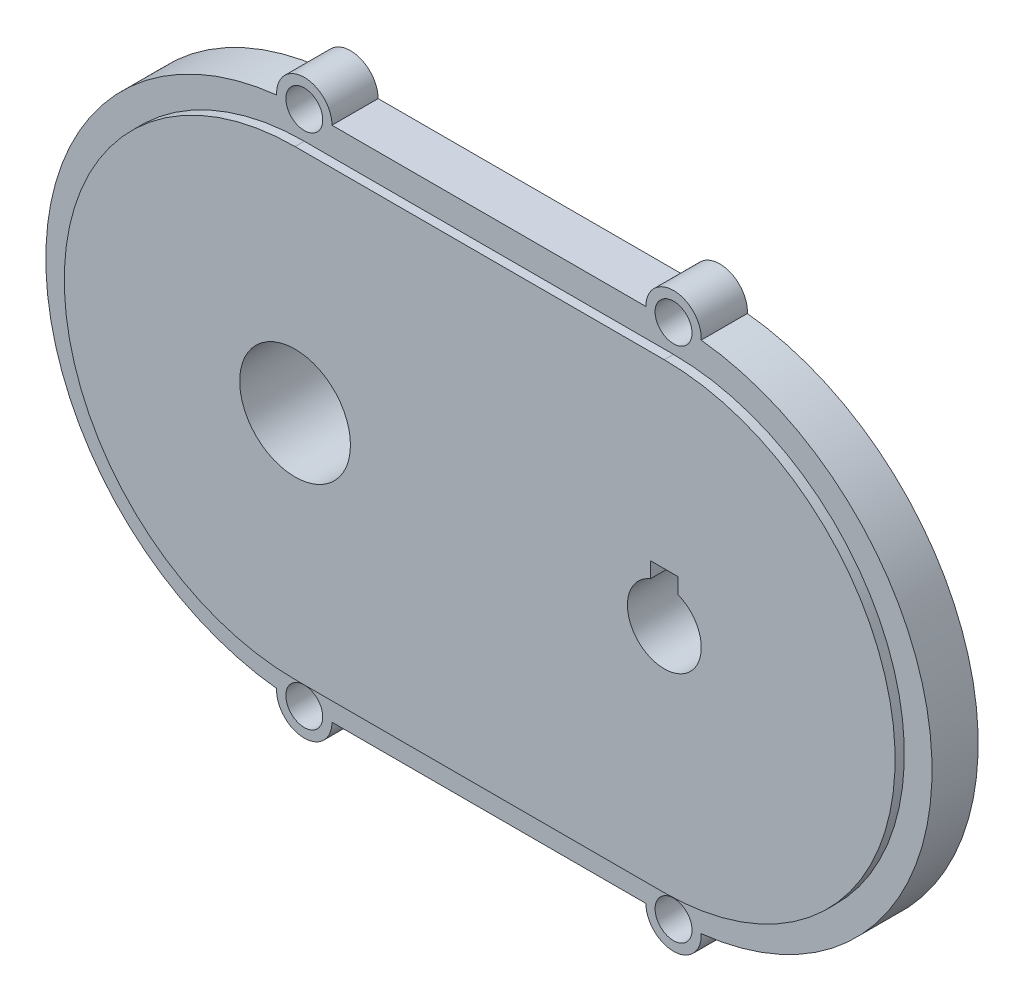
from build123d import *

# Parameters (mm, degrees)
BOSS_EXTRUDE1_DEPTH = 5
BOSS_EXTRUDE2_DEPTH = 1
SKETCH5_R           = 3
BOSS_EXTRUDE3_DEPTH = 5
SKETCH6_R           = 2
CUT_EXTRUDE1_DEPTH  = 5
SKETCH7_R           = 6
SKETCH7_R_2         = 8
BOSS_EXTRUDE4_DEPTH = 8
SKETCH8_R           = 6
SKETCH8_R_2         = 4
CUT_EXTRUDE2_DEPTH  = 11
CUT_EXTRUDE3_DEPTH  = 1.4


with BuildPart() as part:
    # Sketch2 → Boss-Extrude1 (new body)
    with BuildSketch(Plane.XY):
        with BuildLine():
            Line((-20, 28), (20, 28))
            ThreePointArc((20, 28), (48, 0), (20, -28))
            Line((20, -28), (-20, -28))
            ThreePointArc((-20, -28), (-48, 0), (-20, 28))
        make_face()
    extrude(amount=BOSS_EXTRUDE1_DEPTH)

    # Sketch4 → Boss-Extrude2 (add)
    with BuildSketch(Plane.XY.offset(5)):
        with BuildLine():
            Line((-20, 25), (20, 25))
            ThreePointArc((20, 25), (45, 0), (20, -25))
            Line((20, -25), (-20, -25))
            ThreePointArc((-20, -25), (-45, 0), (-20, 25))
        make_face()
    extrude(amount=BOSS_EXTRUDE2_DEPTH)

    # Sketch5 → Boss-Extrude3 (add)
    with BuildSketch(Plane(origin=(0, 0, 0), x_dir=(-1, 0, 0), z_dir=(0, 0, -1))):
        with Locations((-20, 28)):
            Circle(SKETCH5_R)
        with Locations((20, 28)):
            Circle(SKETCH5_R)
        with Locations((-20, -28)):
            Circle(SKETCH5_R)
        with Locations((20, -28)):
            Circle(SKETCH5_R)
    extrude(amount=-BOSS_EXTRUDE3_DEPTH)

    # Sketch6 → Cut-Extrude1 (cut)
    with BuildSketch(Plane(origin=(0, 0, 0), x_dir=(-1, 0, 0), z_dir=(0, 0, -1))):
        with Locations((-20, 28)):
            Circle(SKETCH6_R)
        with Locations((20, 28)):
            Circle(SKETCH6_R)
        with Locations((-20, -28)):
            Circle(SKETCH6_R)
        with Locations((20, -28)):
            Circle(SKETCH6_R)
    extrude(amount=-CUT_EXTRUDE1_DEPTH, mode=Mode.SUBTRACT)

    # Sketch7 → Boss-Extrude4 (add)
    with BuildSketch(Plane(origin=(0, 0, 0), x_dir=(-1, 0, 0), z_dir=(0, 0, -1))):
        with Locations(Location((-20, 0, 0), (0, 0, 180))):
            Circle(SKETCH7_R)
        with Locations(Location((20, 0, 0), (0, 0, 180))):
            Circle(SKETCH7_R_2)
    extrude(amount=BOSS_EXTRUDE4_DEPTH)

    # Sketch8 → Cut-Extrude2 (cut)
    with BuildSketch(Plane.XY.offset(6)):
        with Locations((-20, 0)):
            Circle(SKETCH8_R)
        with Locations((20, 0)):
            Circle(SKETCH8_R_2)
    extrude(amount=-CUT_EXTRUDE2_DEPTH, mode=Mode.SUBTRACT)

    # Sketch9 → Cut-Extrude3 (cut, symmetric)
    with BuildSketch(Plane(origin=(0, 4, 0), x_dir=(1, 0, 0), z_dir=(0, 1, 0))):
        with BuildLine():
            Line((18.5, -7.970089987), (18.5, 1.6))
            ThreePointArc((18.5, 1.6), (20, 3.1), (21.5, 1.6))
            Line((21.5, 1.6), (21.5, -7.970089987))
            ThreePointArc((21.5, -7.970089987), (20, -9.470089987), (18.5, -7.970089987))
        make_face()
    extrude(amount=CUT_EXTRUDE3_DEPTH, both=True, mode=Mode.SUBTRACT)


solid = part.part
